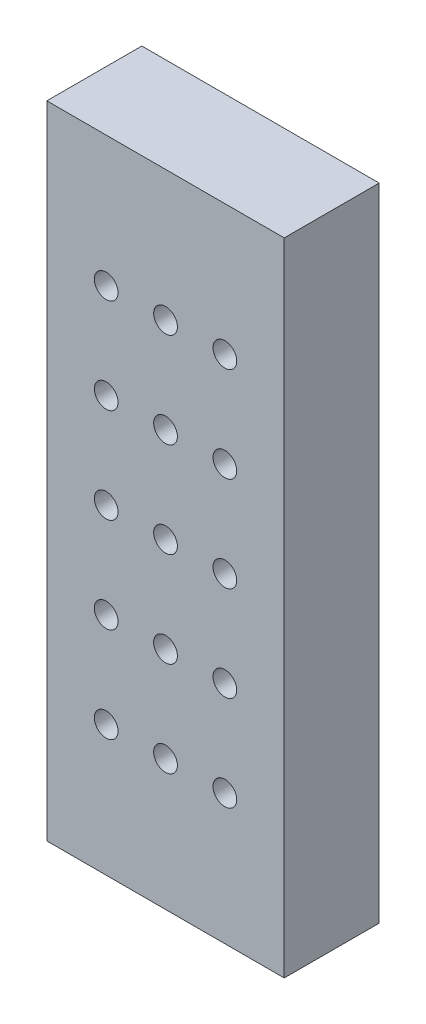
from build123d import *

# Parameters (mm, degrees)
SKETCH_1_W               = 10
SKETCH_1_H               = 27
EXTRUDE_1_DEPTH          = 4
CUT_EXTRUDE_1_REACH      = 16.942
SKETCH_2_R               = 0.5
PATTERN_LINEAR_2_COUNT   = 3
PATTERN_LINEAR_2_PITCH   = 4
MIRROR_1_COPY_1_REACH    = 16.942
MIRROR_1_COPY_1_SKETCH_R = 0.5
MIRROR_1_COPY_2_REACH    = 16.942
MIRROR_1_COPY_2_SKETCH_R = 0.5


with BuildPart() as part:
    # 草图1 → 凸台-拉伸1 (new body)
    with BuildSketch(Plane.XY):
        Rectangle(SKETCH_1_W, SKETCH_1_H)
    extrude(amount=EXTRUDE_1_DEPTH)

    # 草图2 → 切除-拉伸1 (cut, up to next)
    with BuildSketch(Plane.XY.offset(4), mode=Mode.PRIVATE) as cut_extrude_1_sk1:
        Circle(SKETCH_2_R)
    cut_extrude_1_tool1 = extrude(cut_extrude_1_sk1.sketch, amount=-CUT_EXTRUDE_1_REACH, mode=Mode.PRIVATE) & part.part
    # 草图2 → 切除-拉伸1 (cut, up to next)
    with BuildSketch(Plane.XY.offset(4), mode=Mode.PRIVATE) as cut_extrude_1_sk2:
        with Locations((-2.5, 0)):
            Circle(SKETCH_2_R)
    cut_extrude_1_tool2 = extrude(cut_extrude_1_sk2.sketch, amount=-CUT_EXTRUDE_1_REACH, mode=Mode.PRIVATE) & part.part
    # 草图2 → 切除-拉伸1 (cut, up to next)
    with BuildSketch(Plane.XY.offset(4), mode=Mode.PRIVATE) as cut_extrude_1_sk3:
        with Locations((2.5, 0)):
            Circle(SKETCH_2_R)
    cut_extrude_1_tool3 = extrude(cut_extrude_1_sk3.sketch, amount=-CUT_EXTRUDE_1_REACH, mode=Mode.PRIVATE) & part.part
    cut_extrude_1_1 = cut_extrude_1_tool1.solids().sort_by_distance((0, 0, 4))[0]
    add(cut_extrude_1_1, mode=Mode.SUBTRACT)
    cut_extrude_1_2 = cut_extrude_1_tool2.solids().sort_by_distance((-2.5, 0, 4))[0]
    add(cut_extrude_1_2, mode=Mode.SUBTRACT)
    cut_extrude_1_3 = cut_extrude_1_tool3.solids().sort_by_distance((2.5, 0, 4))[0]
    add(cut_extrude_1_3, mode=Mode.SUBTRACT)
    cut_extrude_1 = cut_extrude_1_1 + cut_extrude_1_2 + cut_extrude_1_3  # 切除-拉伸1 as one shape, for the pattern or mirror that repeats it

    # 阵列(线性)2: 切除-拉伸1 ×3
    with Locations(*[(0, -i * PATTERN_LINEAR_2_PITCH, 0) for i in range(1, PATTERN_LINEAR_2_COUNT)]):
        add(cut_extrude_1, mode=Mode.SUBTRACT)

    # 镜向1 copy 1 sketch → 镜向1 copy 1 (cut, up to next)
    with BuildSketch(Plane(origin=(0, 4, 4), x_dir=(1, 0, 0), z_dir=(0, 0, 1)), mode=Mode.PRIVATE) as mirror_1_copy_1_sk1:
        Circle(MIRROR_1_COPY_1_SKETCH_R)
    mirror_1_copy_1_tool1 = extrude(mirror_1_copy_1_sk1.sketch, amount=-MIRROR_1_COPY_1_REACH, mode=Mode.PRIVATE) & part.part
    # 镜向1 copy 1 sketch → 镜向1 copy 1 (cut, up to next)
    with BuildSketch(Plane(origin=(0, 4, 4), x_dir=(1, 0, 0), z_dir=(0, 0, 1)), mode=Mode.PRIVATE) as mirror_1_copy_1_sk2:
        with Locations((-2.5, 0)):
            Circle(MIRROR_1_COPY_1_SKETCH_R)
    mirror_1_copy_1_tool2 = extrude(mirror_1_copy_1_sk2.sketch, amount=-MIRROR_1_COPY_1_REACH, mode=Mode.PRIVATE) & part.part
    # 镜向1 copy 1 sketch → 镜向1 copy 1 (cut, up to next)
    with BuildSketch(Plane(origin=(0, 4, 4), x_dir=(1, 0, 0), z_dir=(0, 0, 1)), mode=Mode.PRIVATE) as mirror_1_copy_1_sk3:
        with Locations((2.5, 0)):
            Circle(MIRROR_1_COPY_1_SKETCH_R)
    mirror_1_copy_1_tool3 = extrude(mirror_1_copy_1_sk3.sketch, amount=-MIRROR_1_COPY_1_REACH, mode=Mode.PRIVATE) & part.part
    add(mirror_1_copy_1_tool1.solids().sort_by_distance((0, 4, 4))[0], mode=Mode.SUBTRACT)
    add(mirror_1_copy_1_tool2.solids().sort_by_distance((-2.5, 4, 4))[0], mode=Mode.SUBTRACT)
    add(mirror_1_copy_1_tool3.solids().sort_by_distance((2.5, 4, 4))[0], mode=Mode.SUBTRACT)

    # 镜向1 copy 2 sketch → 镜向1 copy 2 (cut, up to next)
    with BuildSketch(Plane(origin=(0, 8, 4), x_dir=(1, 0, 0), z_dir=(0, 0, 1)), mode=Mode.PRIVATE) as mirror_1_copy_2_sk1:
        Circle(MIRROR_1_COPY_2_SKETCH_R)
    mirror_1_copy_2_tool1 = extrude(mirror_1_copy_2_sk1.sketch, amount=-MIRROR_1_COPY_2_REACH, mode=Mode.PRIVATE) & part.part
    # 镜向1 copy 2 sketch → 镜向1 copy 2 (cut, up to next)
    with BuildSketch(Plane(origin=(0, 8, 4), x_dir=(1, 0, 0), z_dir=(0, 0, 1)), mode=Mode.PRIVATE) as mirror_1_copy_2_sk2:
        with Locations((-2.5, 0)):
            Circle(MIRROR_1_COPY_2_SKETCH_R)
    mirror_1_copy_2_tool2 = extrude(mirror_1_copy_2_sk2.sketch, amount=-MIRROR_1_COPY_2_REACH, mode=Mode.PRIVATE) & part.part
    # 镜向1 copy 2 sketch → 镜向1 copy 2 (cut, up to next)
    with BuildSketch(Plane(origin=(0, 8, 4), x_dir=(1, 0, 0), z_dir=(0, 0, 1)), mode=Mode.PRIVATE) as mirror_1_copy_2_sk3:
        with Locations((2.5, 0)):
            Circle(MIRROR_1_COPY_2_SKETCH_R)
    mirror_1_copy_2_tool3 = extrude(mirror_1_copy_2_sk3.sketch, amount=-MIRROR_1_COPY_2_REACH, mode=Mode.PRIVATE) & part.part
    add(mirror_1_copy_2_tool1.solids().sort_by_distance((0, 8, 4))[0], mode=Mode.SUBTRACT)
    add(mirror_1_copy_2_tool2.solids().sort_by_distance((-2.5, 8, 4))[0], mode=Mode.SUBTRACT)
    add(mirror_1_copy_2_tool3.solids().sort_by_distance((2.5, 8, 4))[0], mode=Mode.SUBTRACT)


solid = part.part
